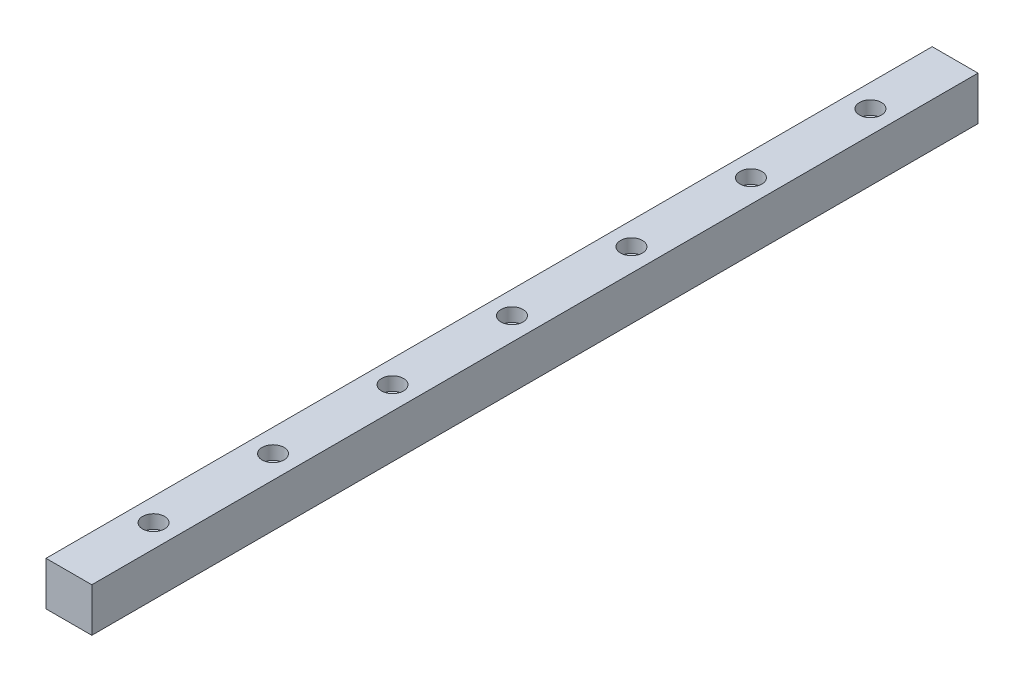
from build123d import *

# Parameters (mm, degrees)
SKETCH_1_W                = 23
SKETCH_1_H                = 22
EXTRUDE_1_DEPTH           = 445
HOLE_WIZARD_1_D           = 6.6
HOLE_WIZARD_1_CBORE_D     = 11
HOLE_WIZARD_1_CBORE_DEPTH = 6.8
PATTERN_LINEAR_1_COUNT    = 8
PATTERN_LINEAR_1_PITCH    = 60


with BuildPart() as part:
    # 草图1 → 凸台-拉伸1 (new body)
    with BuildSketch(Plane.XY):
        with Locations((0, 11)):
            Rectangle(SKETCH_1_W, SKETCH_1_H)
    extrude(amount=EXTRUDE_1_DEPTH)

    # 打孔尺寸(%根据)内六角圆柱头螺钉的类型1 (through all)
    with Locations(Plane(origin=(0, 22, 0), x_dir=(1, 0, 0), z_dir=(0, 1, 0))):
        with Locations((0, -402.5)):
            hole_wizard_1 = CounterBoreHole(HOLE_WIZARD_1_D / 2, HOLE_WIZARD_1_CBORE_D / 2, HOLE_WIZARD_1_CBORE_DEPTH)

    # 阵列(线性)1: 打孔尺寸(%根据)内六角圆柱头螺钉的类型1 ×8
    with Locations(*[(0, 0, -i * PATTERN_LINEAR_1_PITCH) for i in range(1, PATTERN_LINEAR_1_COUNT)]):
        add(hole_wizard_1, mode=Mode.SUBTRACT)


solid = part.part
